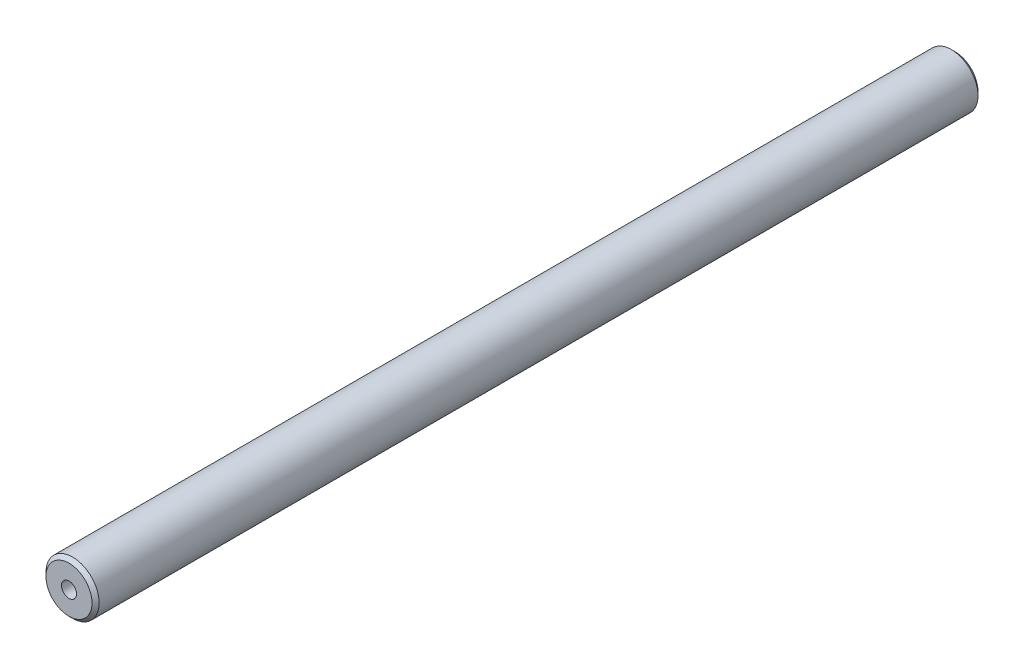
SolidWorks part; units mm, degrees
material "1023 碳钢板 (SS)"
ref_plane "Front Plane" through (0, 0, 0) normal (0, 0, 1) x (1, 0, 0)
ref_plane "Top Plane" through (0, 0, 0) normal (0, 1, 0) x (1, 0, 0)
ref_plane "Right Plane" through (0, 0, 0) normal (1, 0, 0) x (0, 0, -1)
sketch "Sketch1" plane through (0, 0, 0) normal (0, 0, 1) x (1, 0, 0)
  circle A0 centre (0, 0) radius 15
  dimension "D1" = 30
extrude "Boss-Extrude1" add sketch "Sketch1" along normal blind 500
chamfer "Chamfer1" distance 2 angle 45 2 edges at (15, 0, 500) (15, 0, 0)
hole_wizard "M10 Tapped Hole1" positions "Sketch2" profile "Sketch3" tap size "M10" standard "GB"
sketch "Sketch2" plane through (0, 0, 500) normal (0, 0, 1) x (1, 0, 0)
  point P0 (0, 0)
sketch "Sketch3" plane through (0, 0, 500) normal (1, 0, 0) x (0, -1, 0)
  line L0 (0, 0) -> (0, 27.0537)
  line L1 (0, 27.0537) -> (4.25, 24.5)
  line L2 (4.25, 24.5) -> (4.25, 0)
  line L5 (4.25, 0) -> (0, 0)
  line L10 (0, 27.0537) -> (-4.25, 24.5) construction
  line L11 (0, -6.35) -> (0, 107.95) construction
  dimension "螺纹孔钻头直径" = 8.5
  dimension "螺纹孔钻头深度" = 24.5
  dimension "导头角度" = 118
cosmetic thread "CosmeticThread Hole thread1" parameters "D1"=20, "D2"=10
